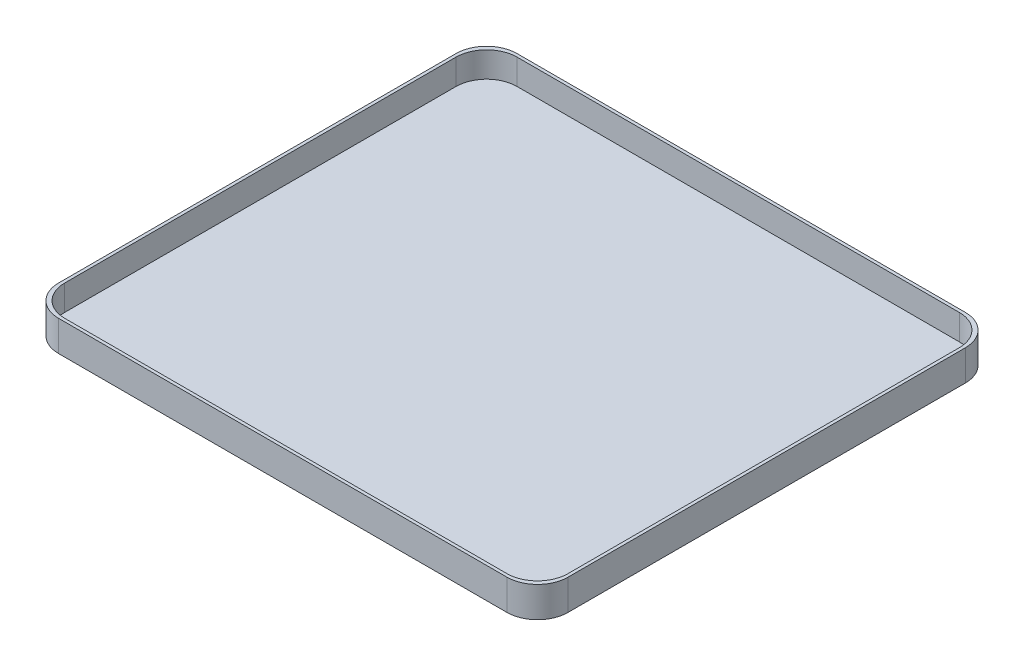
from build123d import *

# Parameters (mm, degrees)
BOSS_EXTRUDE1_DEPTH = 30
CUT_EXTRUDE1_DEPTH  = 25


with BuildPart() as part:
    # Sketch1 → Boss-Extrude1 (new body)
    with BuildSketch(Plane(origin=(0, 0, 0), x_dir=(1, 0, 0), z_dir=(0, 1, 0))):
        with BuildLine():
            Line((-220, 225), (220, 225))
            ThreePointArc((220, 225), (241.213203436, 216.213203436), (250, 195))
            Line((250, 195), (250, -195))
            ThreePointArc((250, -195), (241.213203436, -216.213203436), (220, -225))
            Line((220, -225), (-220, -225))
            ThreePointArc((-220, -225), (-241.213203436, -216.213203436), (-250, -195))
            Line((-250, -195), (-250, 195))
            ThreePointArc((-250, 195), (-241.213203436, 216.213203436), (-220, 225))
        make_face()
    extrude(amount=BOSS_EXTRUDE1_DEPTH)

    # Sketch2 → Cut-Extrude1 (cut)
    with BuildSketch(Plane(origin=(0, 30, 0), x_dir=(1, 0, 0), z_dir=(0, 1, 0))):
        with BuildLine():
            Line((-217, 222), (217, 222))
            ThreePointArc((217, 222), (238.213203436, 213.213203436), (247, 192))
            Line((247, 192), (247, -192))
            ThreePointArc((247, -192), (238.213203436, -213.213203436), (217, -222))
            Line((217, -222), (-217, -222))
            ThreePointArc((-217, -222), (-238.213203436, -213.213203436), (-247, -192))
            Line((-247, -192), (-247, 192))
            ThreePointArc((-247, 192), (-238.213203436, 213.213203436), (-217, 222))
        make_face()
    extrude(amount=-CUT_EXTRUDE1_DEPTH, mode=Mode.SUBTRACT)


solid = part.part
